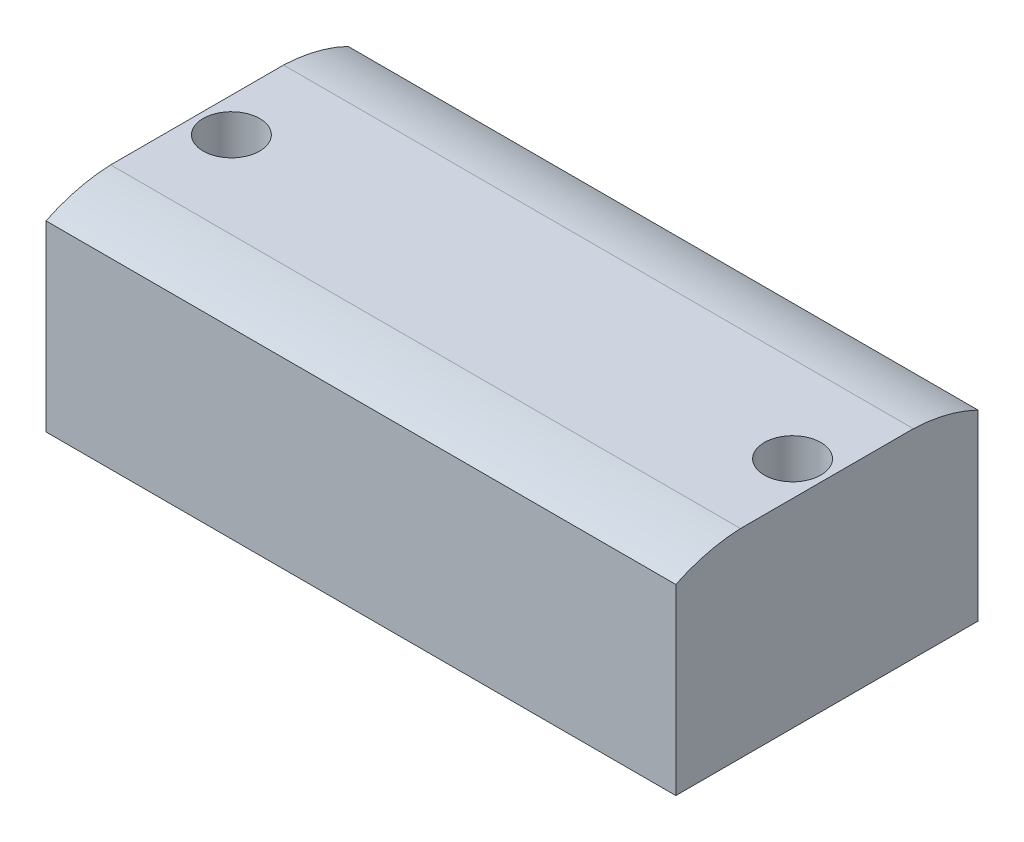
SolidWorks part; units mm, degrees
material "PA（尼龙）"
ref_plane "前视基准面" through (0, 0, 0) normal (0, 0, 1) x (1, 0, 0)
ref_plane "上视基准面" through (0, 0, 0) normal (0, 1, 0) x (1, 0, 0)
ref_plane "右视基准面" through (0, 0, 0) normal (1, 0, 0) x (0, 0, -1)
sketch "草图1" plane through (0, 0, 0) normal (0, 0, 1) x (1, 0, 0)
  line L0 (-28.1102, 0) -> (28.3336, 0) construction
  line L1 (0, 16.2148) -> (0, -17.0358) construction
  line L3 (-38.98, 12.315) -> (38.98, 12.315)
  line L4 (-38.98, 12.315) -> (-38.98, -12.315)
  line L5 (-38.98, -12.315) -> (38.98, -12.315)
  line L6 (38.98, 12.315) -> (38.98, -12.315)
  dimension "D1" = 24.63
  dimension "D2" = 77.96
extrude "凸台-拉伸1" add sketch "草图1" along normal mid plane 37.4
sketch "草图2" plane through (38.98, 0, 0) normal (1, 0, 0) x (0, 0, -1)
  line L0 (-18.7, 10.315) -> (-18.7, 12.315)
  line L1 (-18.7, -12.315) -> (-18.7, 12.315) construction
  line L2 (-18.7, 12.315) -> (-10.7, 12.315)
  line L3 (-18.7, 12.315) -> (18.7, 12.315) construction
  line L4 (0, 12.8817) -> (0, -13.6914) construction
  line L5 (18.7, 12.315) -> (10.7, 12.315)
  line L6 (18.7, 10.315) -> (18.7, 12.315)
  arc A0 (-10.7, 12.315) -> (-18.7, 10.315) centre (-9.9535, -7.6711) ccw
  arc A1 (10.7, 12.315) -> (18.7, 10.315) centre (9.9535, -7.6711) cw
  dimension "D3" = 20
  dimension "D1" = 2
  dimension "D2" = 8
extrude "切除-拉伸1" cut sketch "草图2" against normal through all
sketch "草图3" plane through (0, 12.315, 0) normal (0, 1, 0) x (1, 0, 0)
  line L0 (-60.2814, 0) -> (61.6322, 0) construction
  line L1 (0, 20.1501) -> (0, -23.7523) construction
  circle A0 centre (-34.73, 0) radius 2.05
  circle A1 centre (34.73, 0) radius 2.05
  dimension "D1" = 4.1
  dimension "D2" = 69.46
extrude "切除-拉伸2" cut sketch "草图3" against normal through all
sketch "草图4" plane through (0, 12.315, 0) normal (0, 1, 0) x (1, 0, 0)
  circle A0 centre (-34.73, 0) radius 3.5
  circle A1 centre (34.73, 0) radius 3.5
  dimension "D1" = 7
extrude "切除-拉伸3" cut sketch "草图4" against normal blind 5
